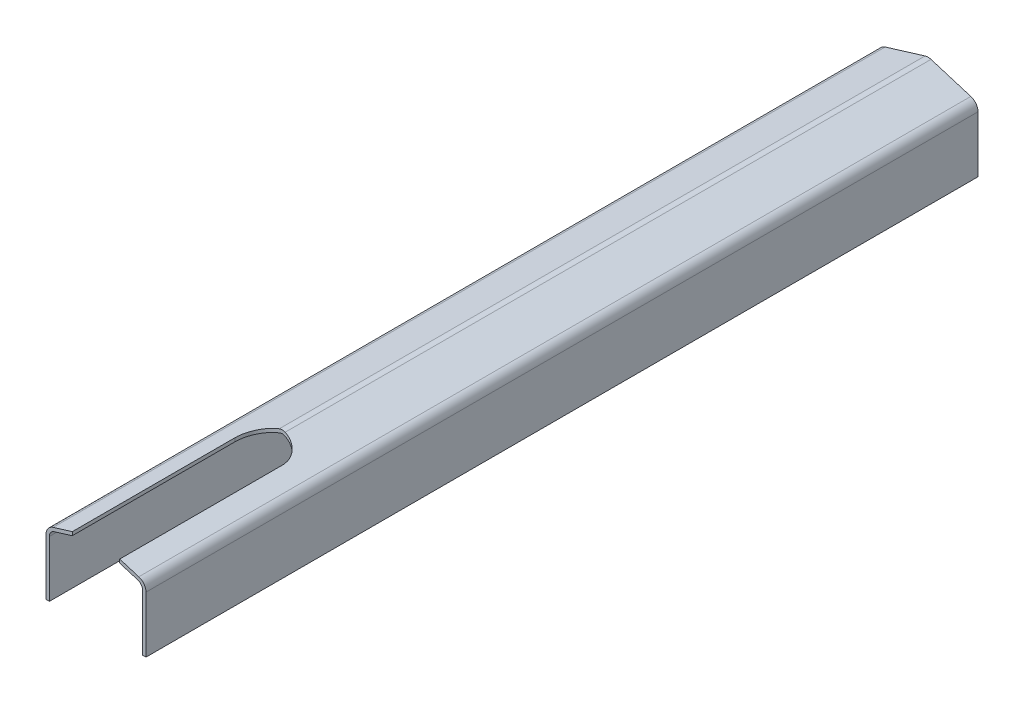
from build123d import *

# Parameters (mm, degrees)
BOSS_EXTRUDE1_DEPTH    = 2455
CUT_EXTRUDE1_DEPTH     = 2471.34516819
CUT_EXTRUDE2_DEPTH     = 10
M10_TAPPED_HOLE1_D     = 8.5
M10_TAPPED_HOLE1_DEPTH = 27.5
M10_TAPPED_HOLE1_TIP   = 2.553657631


with BuildPart() as part:
    # Sketch1 → Boss-Extrude1 (new body)
    with BuildSketch(Plane.XY):
        with BuildLine():
            Line((-147.5, 0), (-147.5, 166.076644929))
            ThreePointArc((-147.5, 166.076644929), (-141.615705819, 183.921328531), (-126.271151142, 194.765787607))
            Line((-126.271151142, 194.765787607), (-8.771151142, 230.689142679))
            ThreePointArc((-8.771151142, 230.689142679), (0, 232), (8.771151142, 230.689142679))
            Line((8.771151142, 230.689142679), (126.271151142, 194.765787607))
            ThreePointArc((126.271151142, 194.765787607), (141.615705819, 183.921328531), (147.5, 166.076644929))
            Line((147.5, 166.076644929), (147.5, 0))
            Line((147.5, 0), (137.5, 0))
            Line((137.5, 0), (137.5, 166.076644929))
            ThreePointArc((137.5, 166.076644929), (133.577137212, 177.973100664), (123.347434094, 185.202740048))
            Line((123.347434094, 185.202740048), (5.847434094, 221.126095119))
            ThreePointArc((5.847434094, 221.126095119), (0, 222), (-5.847434094, 221.126095119))
            Line((-5.847434094, 221.126095119), (-123.347434094, 185.202740048))
            ThreePointArc((-123.347434094, 185.202740048), (-133.577137212, 177.973100664), (-137.5, 166.076644929))
            Line((-137.5, 166.076644929), (-137.5, 0))
            Line((-137.5, 0), (-147.5, 0))
        make_face()
    extrude(amount=BOSS_EXTRUDE1_DEPTH)

    # Sketch2 → Cut-Extrude1 (cut, through all)
    with BuildSketch(Plane(origin=(0, 0, 0), x_dir=(1, 0, 0), z_dir=(0, 1, 0))):
        with BuildLine():
            Line((-70, -1975), (-70, -2455))
            Line((-70, -2455), (70, -2455))
            Line((70, -2455), (70, -1975))
            ThreePointArc((70, -1975), (0, -1905), (-70, -1975))
        make_face()
    extrude(amount=CUT_EXTRUDE1_DEPTH, mode=Mode.SUBTRACT)

    # Sketch3 → Cut-Extrude2 (cut)
    with BuildSketch(Plane.ZY.offset(147.5)):
        with BuildLine():
            Line((1545, 137), (1585, 137))
            ThreePointArc((1585, 137), (1625, 97), (1585, 57))
            Line((1585, 57), (1545, 57))
            ThreePointArc((1545, 57), (1505, 97), (1545, 137))
        make_face()
    extrude(amount=-CUT_EXTRUDE2_DEPTH, mode=Mode.SUBTRACT)

    # M10 Tapped Hole1
    with Locations(Plane.ZY.offset(147.5)):
        with Locations((1565, 147), (1565, 47), (1495, 97), (1635, 97)):
            Hole(M10_TAPPED_HOLE1_D / 2, depth=M10_TAPPED_HOLE1_DEPTH)
            with Locations((0, 0, -(M10_TAPPED_HOLE1_DEPTH + M10_TAPPED_HOLE1_TIP / 2))):  # 118° drill point
                Cone(0, M10_TAPPED_HOLE1_D / 2, M10_TAPPED_HOLE1_TIP, mode=Mode.SUBTRACT)


solid = part.part
